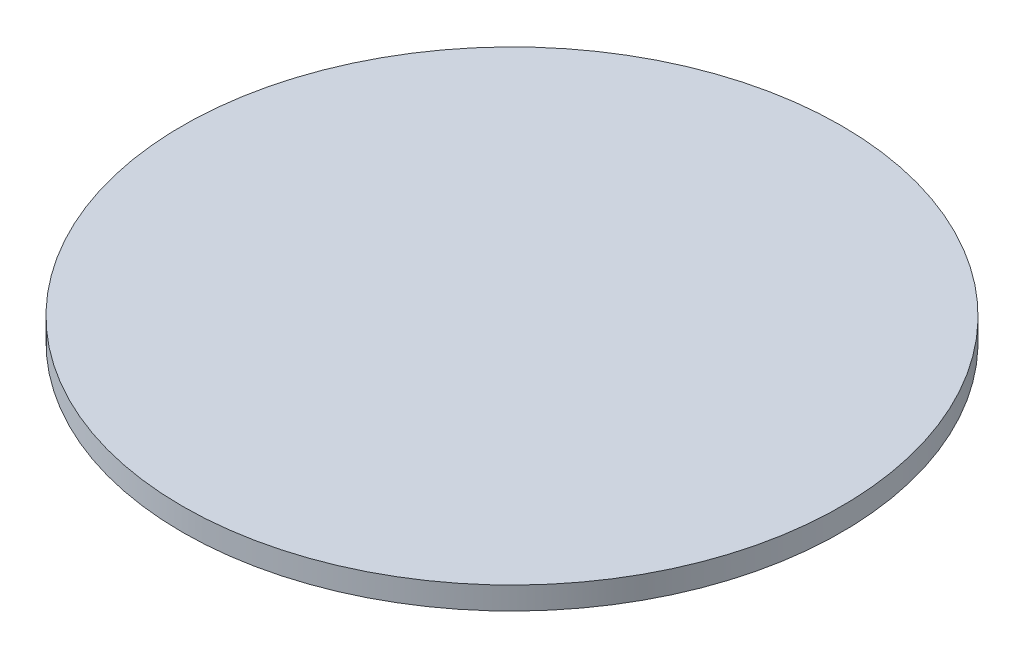
from build123d import *

# Parameters (mm, degrees)
SKETCH_1_W = 29.255663301
SKETCH_1_H = 2


with BuildPart() as part:
    # 草图1 → 旋转1 (revolve)
    with BuildSketch(Plane.XY, mode=Mode.PRIVATE) as revolve_1_sk:
        with Locations((14.627831651, -15.2)):
            Rectangle(SKETCH_1_W, SKETCH_1_H)
    revolve(revolve_1_sk.sketch.rotate(Axis((0, -14.2, 0), (0, 1, 0)), 270), axis=Axis((0, -14.2, 0), (0, 1, 0)))


solid = part.part
